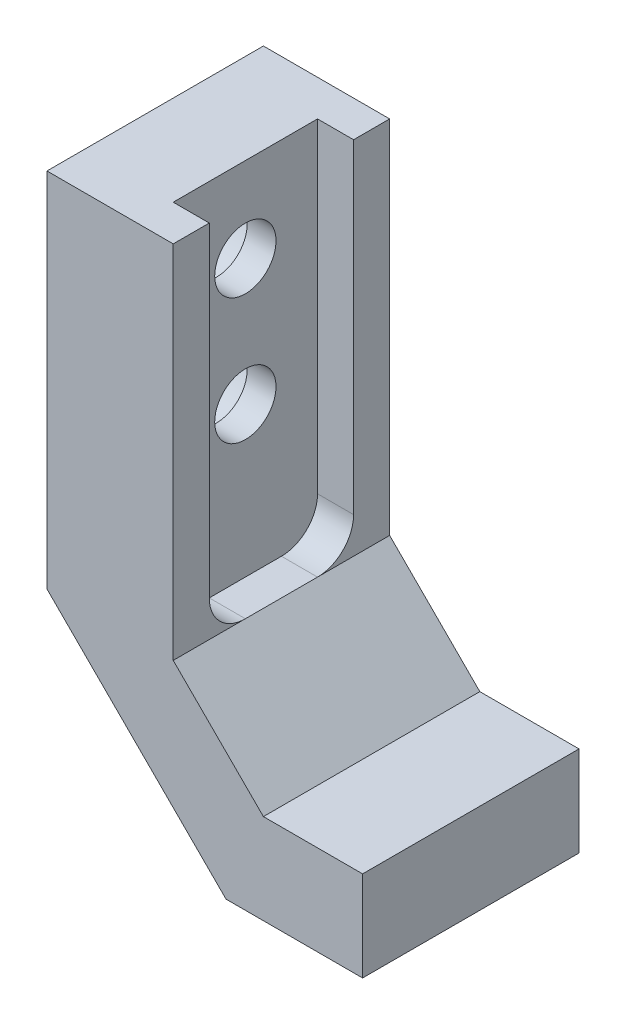
from build123d import *

# Parameters (mm, degrees)
EXTRUDE_1_DEPTH              = 6
SKETCH_2_W                   = 2
SKETCH_2_H                   = 8
CUT_EXTRUDE_1_DEPTH          = 20
FILLET_1_R                   = 2
HOLE_WIZARD_M3_1_D           = 3.4
HOLE_WIZARD_M3_1_CBORE_D     = 6
HOLE_WIZARD_M3_1_CBORE_DEPTH = 3.4


with BuildPart() as part:
    # 草图1 → 凸台-拉伸1 (new, symmetric)
    with BuildSketch(Plane.XY):
        Polygon((0, 0), (0, -20.071067812), (9.928932188, -30), (17.5, -30), (17.5, -25), (12, -25), (7, -20), (7, 0), align=None)
    extrude(amount=EXTRUDE_1_DEPTH, both=True)

    # 草图2 → 切除-拉伸1 (cut)
    with BuildSketch(Plane(origin=(0, 0, 0), x_dir=(1, 0, 0), z_dir=(0, 1, 0))):
        with Locations((6, 0)):
            Rectangle(SKETCH_2_W, SKETCH_2_H)
    extrude(amount=-CUT_EXTRUDE_1_DEPTH, mode=Mode.SUBTRACT)

    # 圆角1
    fillet_1_edges = [part.edges().sort_by_distance(p)[0] for p in [
        (6, -20, 4),
        (6, -20, -4),
    ]]
    fillet(fillet_1_edges, radius=FILLET_1_R)

    # M3 六角圆柱头螺钉的柱形沉头孔1 (through all)
    with Locations(Plane.ZY):
        with Locations((0, -4.7), (0, -11.7)):
            CounterBoreHole(HOLE_WIZARD_M3_1_D / 2, HOLE_WIZARD_M3_1_CBORE_D / 2, HOLE_WIZARD_M3_1_CBORE_DEPTH)


solid = part.part
